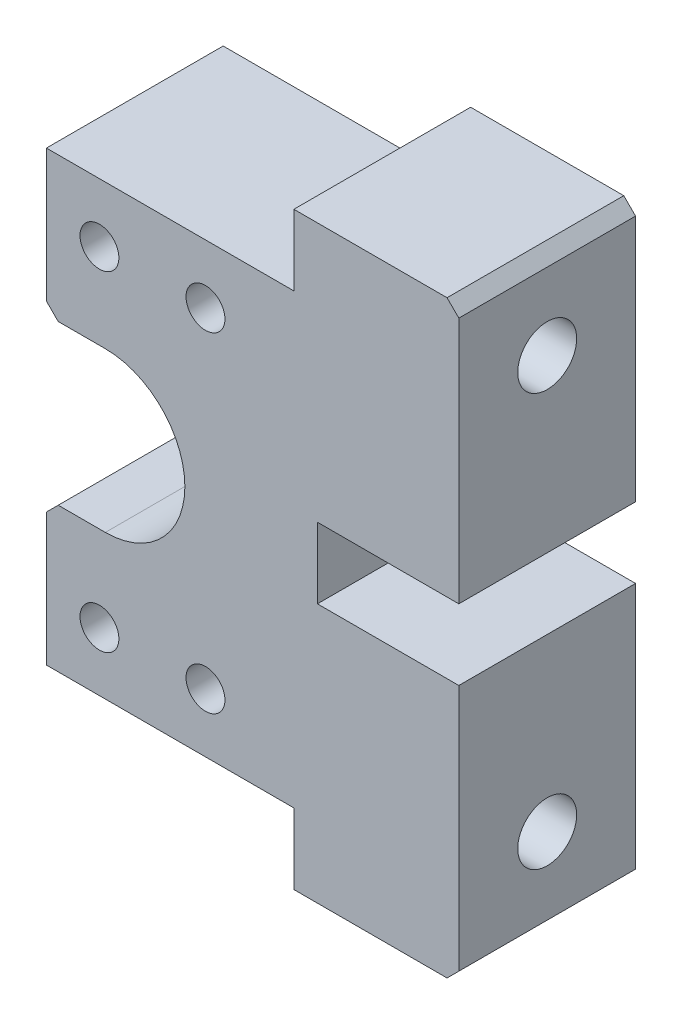
from build123d import *

# Parameters (mm, degrees)
SKETCH_1_W             = 35
SKETCH_1_H             = 50
EXTRUDE_1_DEPTH        = 7.5
CUT_EXTRUDE_1_DEPTH    = 35.003676272
HOLE_WIZARD_M4_2_D     = 3.3
CHAMFER_1_SIZE         = 1
HOLE_WIZARD_M6_1_D     = 5
HOLE_WIZARD_M6_1_DEPTH = 15
HOLE_WIZARD_M6_1_TIP   = 1.502151548
SKETCH_17_W            = 12
SKETCH_17_H            = 6
CUT_EXTRUDE_2_DEPTH    = 35.003676272
SKETCH_19_W            = 21
SKETCH_19_H            = 6
CUT_EXTRUDE_8_DEPTH    = 35.003676272


with BuildPart() as part:
    # 草图1 → 凸台-拉伸1 (new, symmetric)
    with BuildSketch(Plane.XY):
        Rectangle(SKETCH_1_W, SKETCH_1_H)
    extrude(amount=EXTRUDE_1_DEPTH, both=True)

    # 草图2 → 切除-拉伸1 (cut, through all)
    with BuildSketch(Plane.XY.offset(7.5)):
        with BuildLine():
            Line((-17.5, 6.75), (-12.5, 6.75))
            ThreePointArc((-12.5, 6.75), (-5.75, 0), (-12.5, -6.75))
            Line((-12.5, -6.75), (-17.5, -6.75))
            ThreePointArc((-17.5, -6.75), (-24.25, 0), (-17.5, 6.75))
        make_face()
    extrude(amount=-CUT_EXTRUDE_1_DEPTH, mode=Mode.SUBTRACT)

    # M4 螺纹孔2 (through all)
    with Locations(Plane(origin=(0, 0, -7.5), x_dir=(-1, 0, 0), z_dir=(0, 0, -1))):
        with Locations((4, -14), (13, -14), (4, 14), (13, 14)):
            Hole(HOLE_WIZARD_M4_2_D / 2)

    # 倒角1
    chamfer_1_edges = [part.edges().sort_by_distance(p)[0] for p in [
        (-17.5, -6.75, 0),
        (-17.5, 6.75, 0),
        (17.5, -25, 0),
        (17.5, 25, 0),
    ]]
    chamfer(chamfer_1_edges, length=CHAMFER_1_SIZE)

    # M6 螺纹孔1
    with Locations(Plane(origin=(17.5, 0, 0), x_dir=(0, 0, -1), z_dir=(1, 0, 0))):
        with Locations((0, -17.5), (0, 17.5)):
            Hole(HOLE_WIZARD_M6_1_D / 2, depth=HOLE_WIZARD_M6_1_DEPTH)
            with Locations((0, 0, -(HOLE_WIZARD_M6_1_DEPTH + HOLE_WIZARD_M6_1_TIP / 2))):  # 118° drill point
                Cone(0, HOLE_WIZARD_M6_1_D / 2, HOLE_WIZARD_M6_1_TIP, mode=Mode.SUBTRACT)

    # 草图17 → 切除-拉伸2 (cut, through all)
    with BuildSketch(Plane.XY.offset(7.5)):
        with Locations((11.5, 0)):
            Rectangle(SKETCH_17_W, SKETCH_17_H)
    extrude(amount=-CUT_EXTRUDE_2_DEPTH, mode=Mode.SUBTRACT)

    # 草图19 → 切除-拉伸8 (cut, through all)
    with BuildSketch(Plane.XY.offset(7.5)):
        with Locations((-7, -22)):
            Rectangle(SKETCH_19_W, SKETCH_19_H)
        with Locations((-7, 22)):
            Rectangle(SKETCH_19_W, SKETCH_19_H)
    extrude(amount=-CUT_EXTRUDE_8_DEPTH, mode=Mode.SUBTRACT)


solid = part.part
